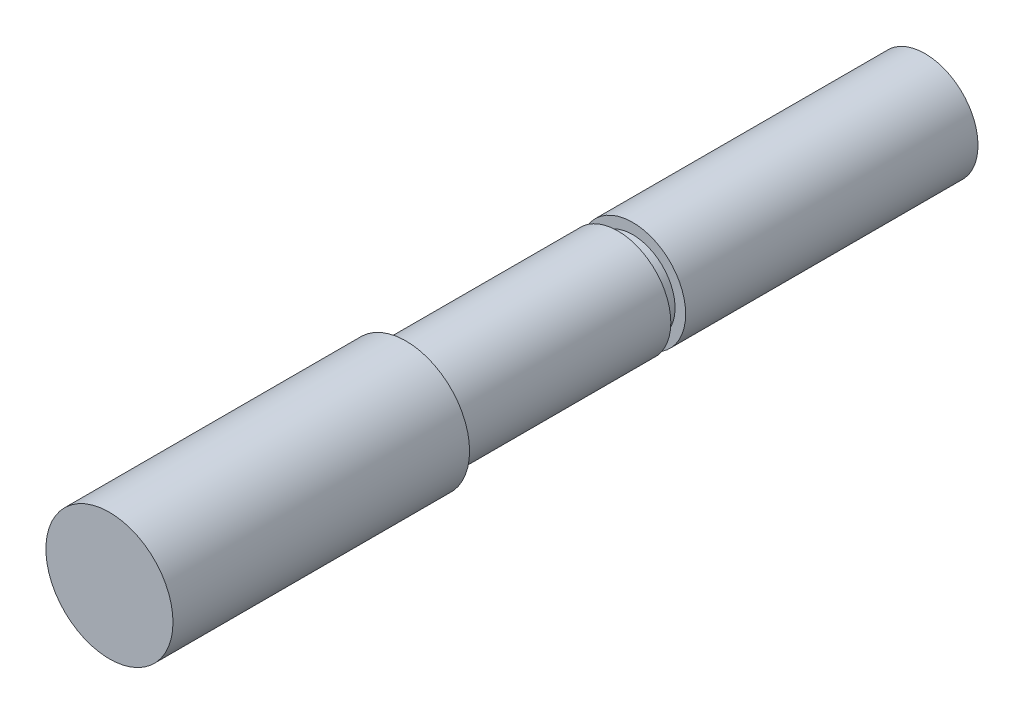
from build123d import *

# Parameters (mm, degrees)
SKETCH_1_R      = 3
EXTRUDE_1_DEPTH = 14
SKETCH_2_R      = 2.5
EXTRUDE_2_DEPTH = 24.5
SKETCH_3_W      = 1.981719741
SKETCH_3_H      = 0.7


with BuildPart() as part:
    # 草图1 → 凸台-拉伸1 (new body)
    with BuildSketch(Plane.XY):
        Circle(SKETCH_1_R)
    extrude(amount=EXTRUDE_1_DEPTH)

    # 草图2 → 凸台-拉伸2 (add)
    with BuildSketch(Plane(origin=(0, 0, 0), x_dir=(-1, 0, 0), z_dir=(0, 0, -1))):
        with Locations(Location((0, 0, 0), (0, 0, 180))):
            Circle(SKETCH_2_R)
    extrude(amount=EXTRUDE_2_DEPTH)

    # 草图3 → 切除-旋转1 (revolve, cut)
    with BuildSketch(Plane(origin=(0, 0, 0), x_dir=(1, 0, 0), z_dir=(0, 1, 0))):
        with Locations((2.990859871, 10.35)):
            Rectangle(SKETCH_3_W, SKETCH_3_H)
    revolve(axis=Axis((0, 0, -21.474636763), (0, 0, 1)), mode=Mode.SUBTRACT)


solid = part.part
